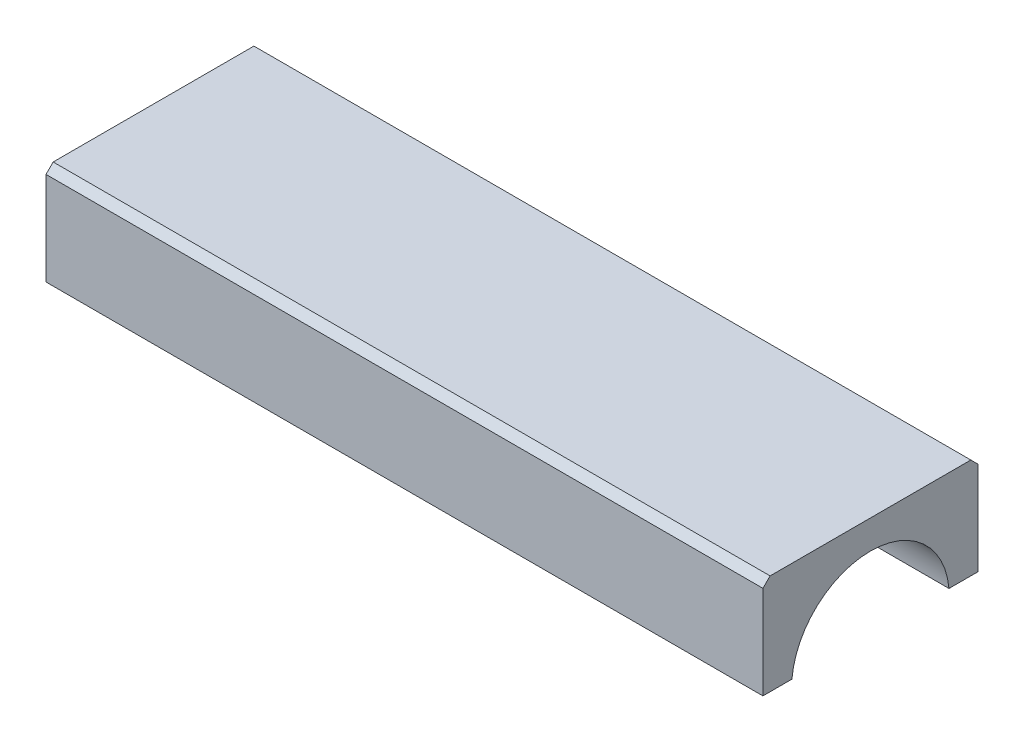
SolidWorks part; units mm, degrees
material "石棉板"
ref_plane "Front Plane" through (0, 0, 0) normal (0, 0, 1) x (1, 0, 0)
ref_plane "Top Plane" through (0, 0, 0) normal (0, 1, 0) x (1, 0, 0)
ref_plane "Right Plane" through (0, 0, 0) normal (1, 0, 0) x (0, 0, -1)
sketch "Sketch1" plane through (0, 0, 0) normal (0, 0, 1) x (1, 0, 0)
  line L1 (-50, 7) -> (50, 7)
  line L2 (-50, 7) -> (-50, -7)
  line L3 (-50, -7) -> (50, -7)
  line L4 (50, 7) -> (50, -7)
  line L5 (-50, 7) -> (50, -7) construction
  line L6 (-50, -7) -> (50, 7) construction
  point P0 (0, 0)
  dimension "D1" = 100
  dimension "D2" = 14
extrude "Boss-Extrude1" add sketch "Sketch1" along normal blind 30
sketch "Sketch2" plane through (-50, 0, 0) normal (-1, 0, 0) x (0, 0, 1)
  line L0 (15, 7) -> (15, -8) construction
  line L1 (30, 7) -> (0, 7) construction
  circle A0 centre (15, -8) radius 11
  dimension "D1" = 15
  dimension "D2" = 22
extrude "Cut-Extrude1" cut sketch "Sketch2" against normal through all
chamfer "Chamfer1" distance 1 angle 45 2 edges at (0, 7, 0) (0, 7, 30)
